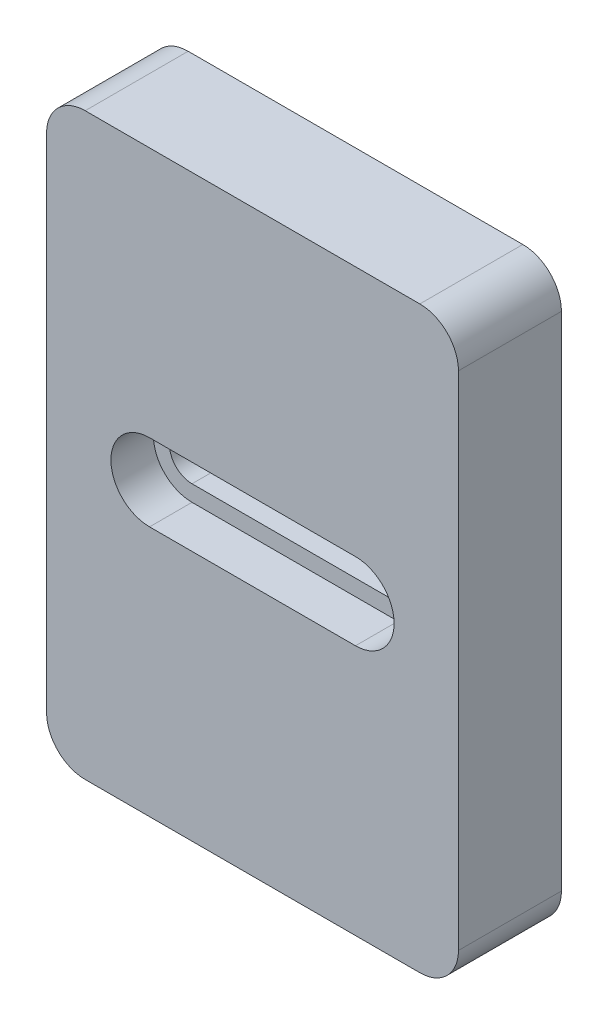
from build123d import *

# Parameters (mm, degrees)
SKETCH1_W           = 32
SKETCH1_H           = 45
BOSS_EXTRUDE1_DEPTH = 8
CUT_EXTRUDE1_DEPTH  = 29.744564704
CUT_EXTRUDE2_DEPTH  = 3.3
FILLET1_R           = 3


with BuildPart() as part:
    # Sketch1 → Boss-Extrude1 (new body)
    with BuildSketch(Plane.XY):
        Rectangle(SKETCH1_W, SKETCH1_H)
    extrude(amount=BOSS_EXTRUDE1_DEPTH)

    # Sketch5 → Cut-Extrude1 (cut, through all)
    with BuildSketch(Plane.XY.offset(8)):
        with BuildLine():
            Line((-8, 1.75), (8, 1.75))
            ThreePointArc((8, 1.75), (9.75, 0), (8, -1.75))
            Line((8, -1.75), (-8, -1.75))
            ThreePointArc((-8, -1.75), (-9.75, 0), (-8, 1.75))
        make_face()
    extrude(amount=-CUT_EXTRUDE1_DEPTH, mode=Mode.SUBTRACT)

    # Sketch6 → Cut-Extrude2 (cut)
    with BuildSketch(Plane.XY.offset(8)):
        with BuildLine():
            Line((-8, 3), (8, 3))
            ThreePointArc((8, 3), (11, 0), (8, -3))
            Line((8, -3), (-8, -3))
            ThreePointArc((-8, -3), (-11, 0), (-8, 3))
        make_face()
    extrude(amount=-CUT_EXTRUDE2_DEPTH, mode=Mode.SUBTRACT)

    # Fillet1
    fillet1_edges = [part.edges().sort_by_distance(p)[0] for p in [
        (-16, 22.5, 4),
        (16, 22.5, 4),
        (16, -22.5, 4),
        (-16, -22.5, 4),
    ]]
    fillet(fillet1_edges, radius=FILLET1_R)


solid = part.part
